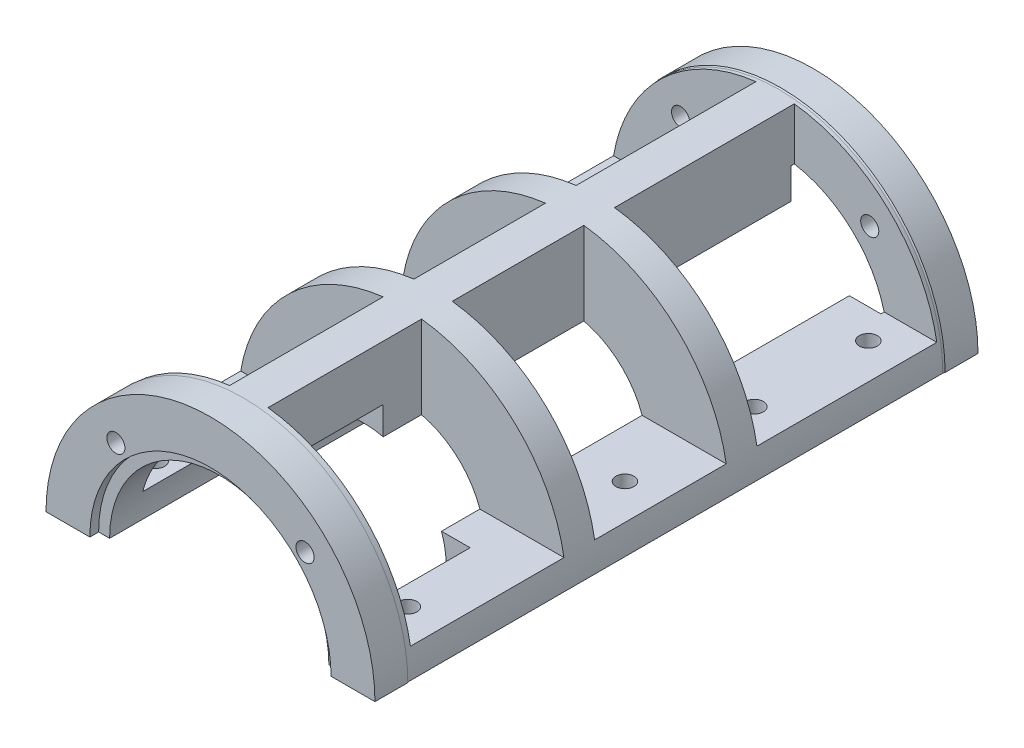
from build123d import *

# Parameters (mm, degrees)
REVOLVE1_ANGLE                   = 180
CUT_EXTRUDE1_DEPTH               = 164
CUT_EXTRUDE2_START               = -164
CUT_EXTRUDE2_DEPTH               = 164
CUT_EXTRUDE3_START               = -140
CUT_EXTRUDE3_DEPTH               = 140
CUT_EXTRUDE4_DEPTH               = 120
CUT_EXTRUDE5_START               = -140
CUT_EXTRUDE5_DEPTH               = 140
CUT_EXTRUDE6_DEPTH               = 120
SKETCH9_W                        = 10.25
SKETCH9_H                        = 350
SKETCH10_W                       = 10.25
SKETCH10_H                       = 350
F_16_5_16_5_DIAMETER_HOLE1_D     = 16.5
F_16_5_16_5_DIAMETER_HOLE2_D     = 16.5
F_16_5_16_5_DIAMETER_HOLE2_DEPTH = 35
F_16_5_16_5_DIAMETER_HOLE3_D     = 16.5
F_16_5_16_5_DIAMETER_HOLE3_DEPTH = 35


with BuildPart() as part:
    # Sketch1 → Revolve1 (revolve)
    with BuildSketch(Plane.XZ.offset(-234.743963655)):
        with BuildLine():
            Line((371.230642584, -1070.692981355), (521.230642584, -1070.692981355))
            Line((521.230642584, -1070.692981355), (521.230642584, -520.692981355))
            Line((521.230642584, -520.692981355), (371.230642584, -520.692981355))
            Line((371.230642584, -520.692981355), (371.230642584, -550.692981355))
            Line((371.230642584, -550.692981355), (371.730642584, -550.692981355))
            Line((371.730642584, -550.692981355), (371.730642584, -1039.03466896))
            ThreePointArc((371.730642584, -1039.03466896), (371.602923908, -1039.900694364), (371.230642584, -1040.692981355))
            Line((371.230642584, -1040.692981355), (371.230642584, -1070.692981355))
        make_face()
    revolve(axis=Axis((521.230642584, 234.743963655, -1070.692981355), (0, 0, -1)), revolution_arc=REVOLVE1_ANGLE)

    # Sketch2 → Cut-Extrude1 (cut)
    with BuildSketch(Plane(origin=(0, 0, -1035.692981355), x_dir=(-1, 0, 0), z_dir=(0, 0, -1))):
        with BuildLine():
            Line((-503.730642584, 383.216183278), (-503.730642584, 259.743963655))
            Line((-503.730642584, 259.743963655), (-373.83576479, 259.743963655))
            ThreePointArc((-373.83576479, 259.743963655), (-418.23099484, 343.10134718), (-503.730642584, 383.216183278))
        make_face()
    extrude(amount=-CUT_EXTRUDE1_DEPTH, mode=Mode.SUBTRACT)

    # Sketch3 → Cut-Extrude2 (cut)
    with BuildSketch(Plane.XY.offset(-871.692981355).offset(CUT_EXTRUDE2_START)):
        with BuildLine():
            Line((538.730642584, 383.216183278), (538.730642584, 259.743963655))
            Line((538.730642584, 259.743963655), (668.625520379, 259.743963655))
            ThreePointArc((668.625520379, 259.743963655), (624.230290328, 343.10134718), (538.730642584, 383.216183278))
        make_face()
    extrude(amount=CUT_EXTRUDE2_DEPTH, mode=Mode.SUBTRACT)

    # Sketch4 → Cut-Extrude3 (cut)
    with BuildSketch(Plane.XY.offset(-555.692981355).offset(CUT_EXTRUDE3_START)):
        with BuildLine():
            Line((503.730642584, 259.743963655), (503.730642584, 383.216183278))
            ThreePointArc((503.730642584, 383.216183278), (418.23099484, 343.10134718), (373.83576479, 259.743963655))
            Line((373.83576479, 259.743963655), (503.730642584, 259.743963655))
        make_face()
    extrude(amount=CUT_EXTRUDE3_DEPTH, mode=Mode.SUBTRACT)

    # Sketch5 → Cut-Extrude4 (cut)
    with BuildSketch(Plane(origin=(0, 0, -843.692981355), x_dir=(-1, 0, 0), z_dir=(0, 0, -1))):
        with BuildLine():
            Line((-503.730642584, 259.743963655), (-373.83576479, 259.743963655))
            ThreePointArc((-373.83576479, 259.743963655), (-418.23099484, 343.10134718), (-503.730642584, 383.216183278))
            Line((-503.730642584, 383.216183278), (-503.730642584, 259.743963655))
        make_face()
    extrude(amount=-CUT_EXTRUDE4_DEPTH, mode=Mode.SUBTRACT)

    # Sketch6 → Cut-Extrude5 (cut)
    with BuildSketch(Plane.XY.offset(-555.692981355).offset(CUT_EXTRUDE5_START)):
        with BuildLine():
            Line((538.730642584, 259.743963655), (668.625520379, 259.743963655))
            ThreePointArc((668.625520379, 259.743963655), (624.230290328, 343.10134718), (538.730642584, 383.216183278))
            Line((538.730642584, 383.216183278), (538.730642584, 259.743963655))
        make_face()
    extrude(amount=CUT_EXTRUDE5_DEPTH, mode=Mode.SUBTRACT)

    # Sketch7 → Cut-Extrude6 (cut)
    with BuildSketch(Plane(origin=(0, 0, -843.692981355), x_dir=(-1, 0, 0), z_dir=(0, 0, -1))):
        with BuildLine():
            Line((-538.730642584, 259.743963655), (-538.730642584, 383.216183278))
            ThreePointArc((-538.730642584, 383.216183278), (-624.230290328, 343.10134718), (-668.625520379, 259.743963655))
            Line((-668.625520379, 259.743963655), (-538.730642584, 259.743963655))
        make_face()
    extrude(amount=-CUT_EXTRUDE6_DEPTH, mode=Mode.SUBTRACT)

    # Sketch8 → Cut-Revolve1 (revolve, cut)
    with BuildSketch(Plane.XZ.offset(-234.743963655)):
        Polygon((631.230642584, -520.692981355), (521.230642584, -520.692981355), (521.230642584, -1070.692981355), (631.230642584, -1070.692981355), (631.230642584, -1062.692981355), (623.730642584, -1062.692981355), (623.730642584, -1032.692981355), (596.230642584, -1032.692981355), (596.230642584, -660.692981355), (621.230642584, -660.692981355), (621.230642584, -528.692981355), (631.230642584, -528.692981355), align=None)
    revolve(axis=Axis((521.230642584, 234.743963655, -520.692981355), (0, 0, -1)), mode=Mode.SUBTRACT)

    # Sketch9 → Cut-Revolve2 (revolve, cut)
    with BuildSketch(Plane.XZ.offset(-234.743963655)):
        with Locations((619.355642584, -847.692981355)):
            Rectangle(SKETCH9_W, SKETCH9_H)
    revolve(axis=Axis((614.230642584, 234.743963655, -672.692981355), (0, 0, -1)), mode=Mode.SUBTRACT)

    # Sketch10 → Cut-Revolve3 (revolve, cut)
    with BuildSketch(Plane.XZ.offset(-234.743963655)):
        with Locations((433.355642584, -847.692981355)):
            Rectangle(SKETCH10_W, SKETCH10_H)
    revolve(axis=Axis((428.230642584, 234.743963655, -672.692981355), (0, 0, -1)), mode=Mode.SUBTRACT)

    # Ø16.5 (16.5) diameter hole1 (through all)
    with Locations(Plane(origin=(0, 259.743963655, 0), x_dir=(1, 0, 0), z_dir=(0, 1, 0))):
        with Locations((636.230642584, 1005.692981355), (636.230642584, 901.692981355), (636.230642584, 783.692981355), (636.230642584, 585.692981355), (406.230642584, 1005.692981355), (406.230642584, 901.692981355), (406.230642584, 585.692981355), (406.230642584, 783.692981355)):
            Hole(F_16_5_16_5_DIAMETER_HOLE1_D / 2)

    # Ø16.5 (16.5) diameter hole2
    with Locations(Plane.XY.offset(-1035.692981355)):
        with Locations((607.497669889, 321.010990959), (434.96361528, 321.010990959)):
            Hole(F_16_5_16_5_DIAMETER_HOLE2_D / 2, depth=F_16_5_16_5_DIAMETER_HOLE2_DEPTH)

    # Ø16.5 (16.5) diameter hole3
    with Locations(Plane(origin=(0, 0, -555.692981355), x_dir=(-1, 0, 0), z_dir=(0, 0, -1))):
        with Locations((-607.497669889, 321.010990959), (-434.96361528, 321.010990959)):
            Hole(F_16_5_16_5_DIAMETER_HOLE3_D / 2, depth=F_16_5_16_5_DIAMETER_HOLE3_DEPTH)


solid = part.part
